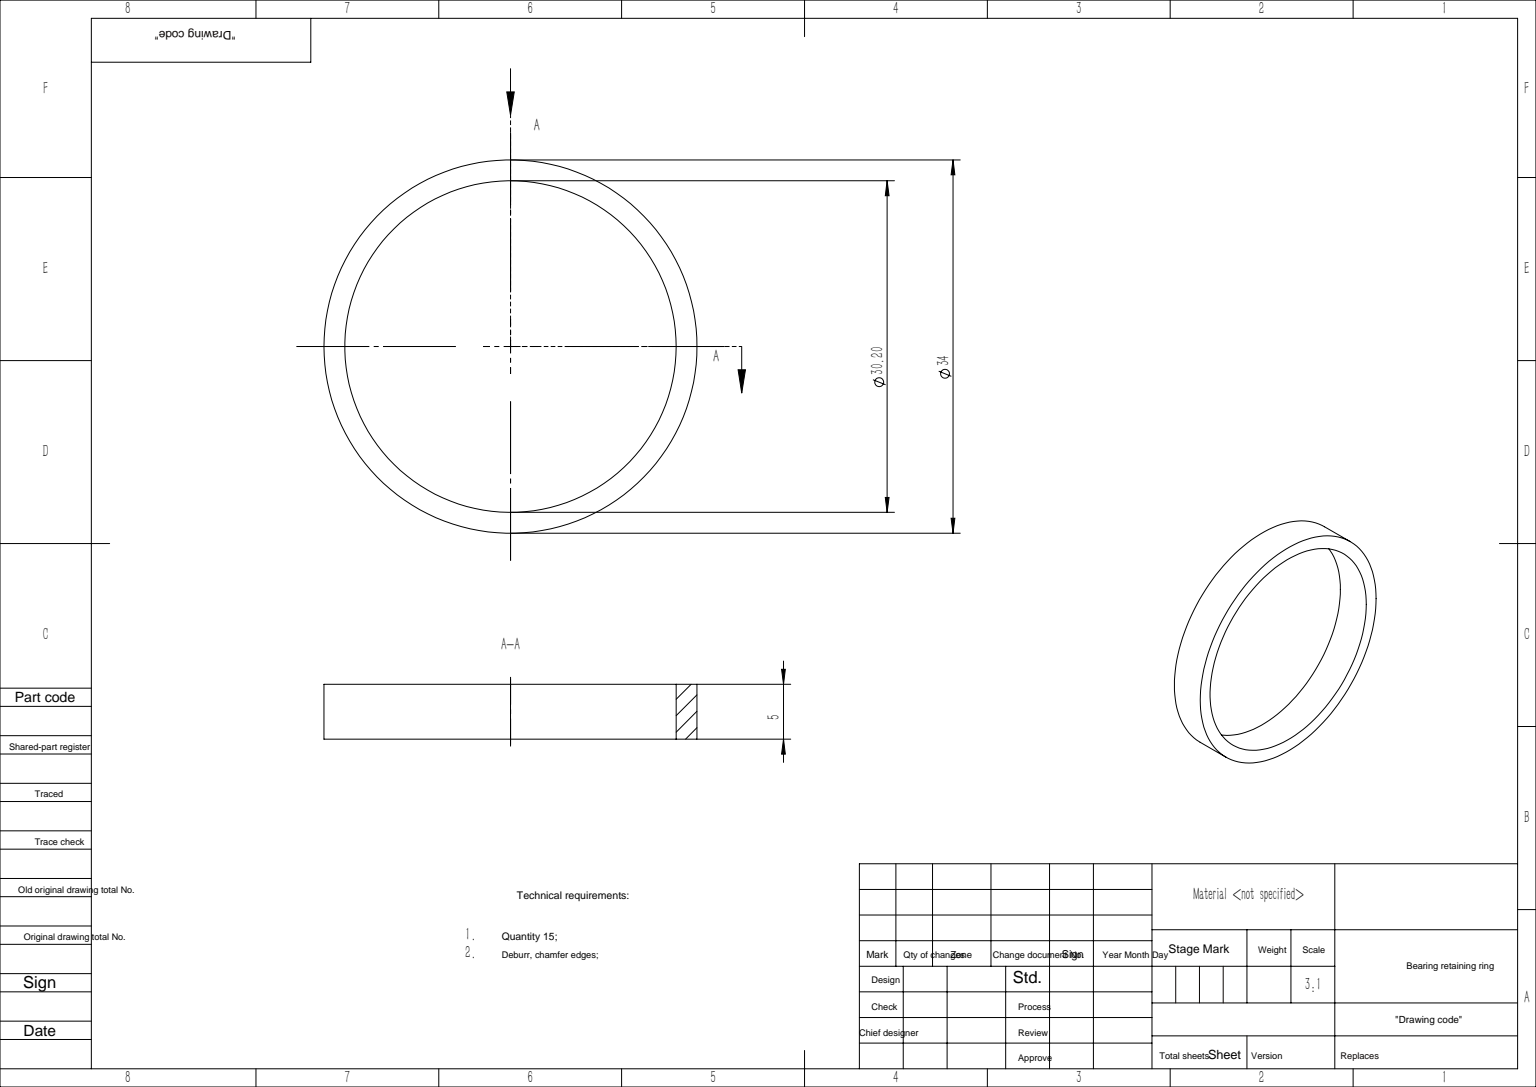
SolidWorks part; units mm, degrees
ref_plane "前视基准面" through (0, 0, 0) normal (0, 0, 1) x (1, 0, 0)
ref_plane "上视基准面" through (0, 0, 0) normal (0, 1, 0) x (1, 0, 0)
ref_plane "右视基准面" through (0, 0, 0) normal (1, 0, 0) x (0, 0, -1)
sketch "草图1" plane through (0, 0, 0) normal (1, 0, 0) x (0, 0, -1)
  circle A0 centre (0, 0) radius 15.1
  circle A1 centre (0, 0) radius 17
  dimension "D1" = 34
  dimension "D2" = 30.2
extrude "凸台-拉伸1" add sketch "草图1" along normal blind 5
